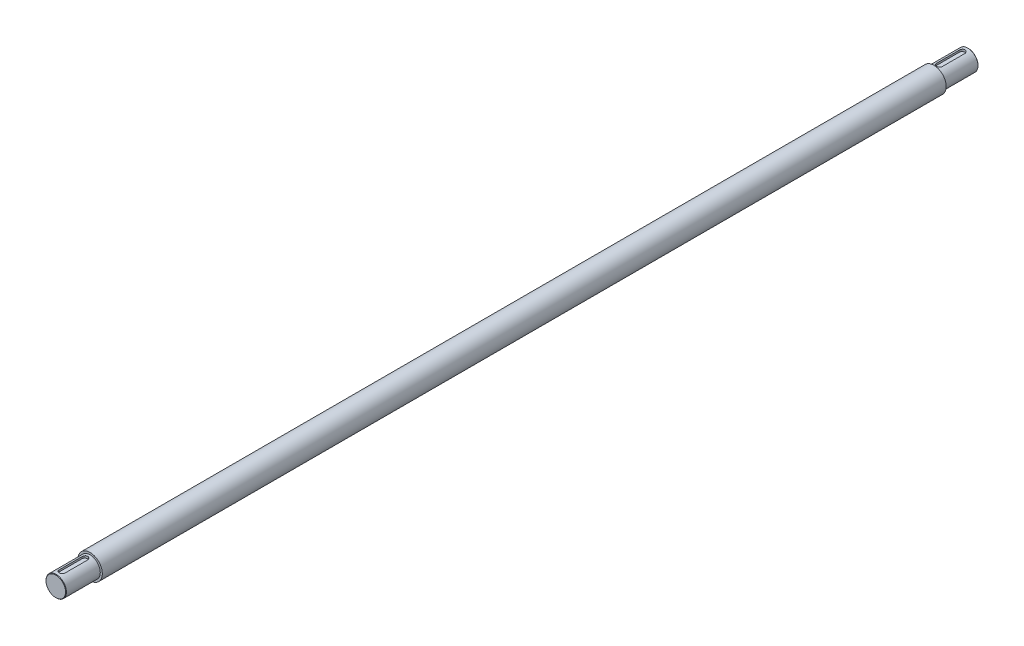
SolidWorks part; units mm, degrees
material "普通碳钢"
ref_plane "Front Plane" through (0, 0, 0) normal (0, 0, 1) x (1, 0, 0)
ref_plane "Top Plane" through (0, 0, 0) normal (0, 1, 0) x (1, 0, 0)
ref_plane "Right Plane" through (0, 0, 0) normal (1, 0, 0) x (0, 0, -1)
sketch "Sketch1" plane through (0, 0, 0) normal (0, 0, 1) x (1, 0, 0)
  circle A0 centre (0, 0) radius 30
  dimension "D1" = 60
extrude "Extrude1" add sketch "Sketch1" along normal mid plane 2067
sketch "Sketch2" plane through (0, 0, 1033.5) normal (0, 0, 1) x (1, 0, 0)
  circle A0 centre (0, 0) radius 25
  dimension "D1" = 50
extrude "Extrude2" add sketch "Sketch2" along normal blind 84
chamfer "Chamfer1" distance 1 angle 45 1 edges at (25, 0, 1117.5)
ref_plane "Plane1" through (0, 19.5, 0) normal (0, 1, 0) x (-1, 0, 0)
sketch "Sketch3" plane through (0, 19.5, 0) normal (0, 1, 0) x (-1, 0, 0)
  line L0 (24, 1117.5) -> (-24, 1117.5) construction
  line L4 (7, 1102.5) -> (7, 1046.5)
  line L11 (-7, 1046.5) -> (-7, 1102.5)
  arc A0 (7, 1046.5) -> (-7, 1046.5) centre (0, 1046.5) cw
  arc A1 (-7, 1102.5) -> (7, 1102.5) centre (0, 1102.5) cw
  dimension "D1" = 7
  dimension "D2" = 7
  dimension "D3" = 15
  dimension "D4" = 56
extrude "Extrude3" cut sketch "Sketch3" along normal blind 5.5
mirror "Mirror1" about plane through (0, 0, 0) normal (0, 0, 1) of "Extrude2", "Chamfer1", "Extrude3"
